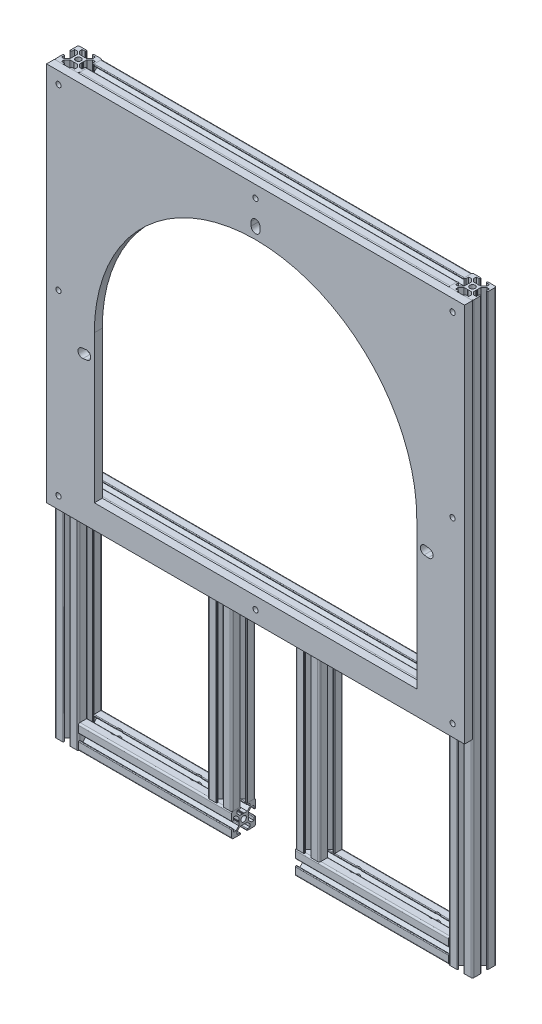
SolidWorks part; units mm, degrees
material "6061 合金"
ref_plane "前视基准面" through (0, 0, 0) normal (0, 0, 1) x (1, 0, 0)
ref_plane "上视基准面" through (0, 0, 0) normal (0, 1, 0) x (1, 0, 0)
ref_plane "右视基准面" through (0, 0, 0) normal (1, 0, 0) x (0, 0, -1)
sketch "草图2" plane through (0, 0, 0) normal (0, 0, 1) x (1, 0, 0)
  line L0 (0, 120) -> (0, 0) construction
  line L1 (262.5, 382.5) -> (-262.5, 382.5)
  line L2 (262.5, 382.5) -> (262.5, -600)
  line L3 (262.5, -600) -> (-262.5, -600)
  line L4 (-262.5, 382.5) -> (-262.5, -600)
  line L5 (0, 0) -> (-79.5734, 0) construction
  line L6 (-184, -30) -> (184, -30)
  line L7 (-184, -30) -> (-184, -525)
  line L8 (184, -30) -> (184, -525)
  circle A5 centre (0, 120) radius 242.5
  circle A6 centre (0, 120) radius 262.5
  point P7 (0, -600)
  dimension "D1" = 485
  dimension "D2" = 184
  dimension "D3" = 525
  dimension "D4" = 120
  dimension "D10" = 30
  dimension "D12" = 600
sketch "草图3" plane through (0, 0, 0) normal (0, 0, 1) x (1, 0, 0)
  line L0 (-247.5, -340) -> (-55, -340)
  line L1 (-247.5, 367.5) -> (247.5, 367.5)
  line L2 (-247.5, 367.5) -> (-247.5, -340)
  line L3 (-247.5, -80) -> (247.5, -80)
  line L4 (247.5, 367.5) -> (247.5, -340)
  line L5 (-55, -80) -> (-55, -340)
  line L6 (0, -22) -> (0, 22) construction
  line L7 (262.5, 382.5) -> (-262.5, 382.5) construction
  line L8 (262.5, 382.5) -> (262.5, -600) construction
  line L9 (-184, -30) -> (184, -30) construction
  line L10 (55, -80) -> (55, -340)
  line L11 (55, -340) -> (247.5, -340)
  point P8 (0, 367.5)
  dimension "D1" = 50
  dimension "D2" = 15
  dimension "D3" = 15
  dimension "D4" = 260
  dimension "D5" = 110
other "铝型材 30 X 30 X R2(1)"
ref_plane "基准面1" through (-247.5, 367.5, 0) normal (0, -1, 0) x (1, 0, 0)
sketch "草图1" plane through (-247.5, 367.5, 0) normal (0, -1, 0) x (1, 0, 0)
  line L0 (-15, -4.8) -> (-15, -13)
  line L1 (-13, -15) -> (-4.8, -15)
  line L2 (-4, -14.2) -> (-4, -13.8)
  line L3 (-4.8, -13) -> (-8.25, -13)
  line L4 (-8.25, -13) -> (-8.25, -9.6642)
  line L5 (-8.25, -9.6642) -> (-4.5858, -6)
  line L6 (-4.5858, -6) -> (-0.6536, -6)
  line L7 (-0.4036, -5.933) -> (0, -5.7)
  line L8 (0, -5.7) -> (0.4036, -5.933)
  line L9 (0.9036, -5.933) -> (1.2189, -5.751)
  line L10 (1.2189, -5.751) -> (2.5, -6)
  line L11 (2.5, -6) -> (4.5858, -6)
  line L12 (4.5858, -6) -> (8.25, -9.6642)
  line L13 (8.25, -9.6642) -> (8.25, -13)
  line L14 (8.25, -13) -> (4.8, -13)
  line L15 (4, -13.8) -> (4, -14.2)
  line L16 (4.8, -15) -> (13, -15)
  line L17 (15, -13) -> (15, -4.8)
  line L18 (14.2, -4) -> (13.8, -4)
  line L19 (13, -4.8) -> (13, -8.25)
  line L20 (13, -8.25) -> (9.6642, -8.25)
  line L21 (9.6642, -8.25) -> (6, -4.5858)
  line L22 (6, -4.5858) -> (6, -0.6536)
  line L23 (5.933, -0.4036) -> (5.7, 0)
  line L24 (5.7, 0) -> (5.933, 0.4036)
  line L25 (5.933, 0.9036) -> (5.751, 1.2189)
  line L26 (5.751, 1.2189) -> (6, 2.5)
  line L27 (6, 2.5) -> (6, 4.5858)
  line L28 (6, 4.5858) -> (9.6642, 8.25)
  line L29 (9.6642, 8.25) -> (13, 8.25)
  line L30 (13, 8.25) -> (13, 4.8)
  line L31 (13.8, 4) -> (14.2, 4)
  line L32 (15, 4.8) -> (15, 13)
  line L33 (13, 15) -> (4.8, 15)
  line L34 (4, 14.2) -> (4, 13.8)
  line L35 (4.8, 13) -> (8.25, 13)
  line L36 (8.25, 13) -> (8.25, 9.6642)
  line L37 (8.25, 9.6642) -> (4.5858, 6)
  line L38 (4.5858, 6) -> (0.6536, 6)
  line L39 (0.4036, 5.933) -> (0, 5.7)
  line L40 (0, 5.7) -> (-0.4036, 5.933)
  line L41 (-0.9036, 5.933) -> (-1.2189, 5.751)
  line L42 (-1.2189, 5.751) -> (-2.5, 6)
  line L43 (-2.5, 6) -> (-4.5858, 6)
  line L44 (-4.5858, 6) -> (-8.25, 9.6642)
  line L45 (-8.25, 9.6642) -> (-8.25, 13)
  line L46 (-8.25, 13) -> (-4.8, 13)
  line L47 (-4, 13.8) -> (-4, 14.2)
  line L48 (-4.8, 15) -> (-13, 15)
  line L49 (-15, 13) -> (-15, 4.8)
  line L50 (-14.2, 4) -> (-13.8, 4)
  line L51 (-13, 4.8) -> (-13, 8.25)
  line L52 (-13, 8.25) -> (-9.6642, 8.25)
  line L53 (-9.6642, 8.25) -> (-6, 4.5858)
  line L54 (-6, 4.5858) -> (-6, 0.6536)
  line L55 (-5.933, 0.4036) -> (-5.7, 0)
  line L56 (-5.7, 0) -> (-5.933, -0.4036)
  line L57 (-5.933, -0.9036) -> (-5.751, -1.2189)
  line L58 (-5.751, -1.2189) -> (-6, -2.5)
  line L59 (-6, -2.5) -> (-6, -4.5858)
  line L60 (-6, -4.5858) -> (-9.6642, -8.25)
  line L61 (-9.6642, -8.25) -> (-13, -8.25)
  line L62 (-13, -8.25) -> (-13, -4.8)
  line L63 (-13.8, -4) -> (-14.2, -4)
  arc A0 (-15, -13) -> (-13, -15) centre (-13, -13) ccw
  arc A1 (-4.8, -15) -> (-4, -14.2) centre (-4.8, -14.2) ccw
  arc A2 (-4, -13.8) -> (-4.8, -13) centre (-4.8, -13.8) ccw
  arc A3 (-0.6536, -6) -> (-0.4036, -5.933) centre (-0.6536, -5.5) ccw
  arc A4 (0.4036, -5.933) -> (0.9036, -5.933) centre (0.6536, -5.5) ccw
  arc A5 (4.8, -13) -> (4, -13.8) centre (4.8, -13.8) ccw
  arc A6 (4, -14.2) -> (4.8, -15) centre (4.8, -14.2) ccw
  arc A7 (13, -15) -> (15, -13) centre (13, -13) ccw
  arc A8 (15, -4.8) -> (14.2, -4) centre (14.2, -4.8) ccw
  arc A9 (13.8, -4) -> (13, -4.8) centre (13.8, -4.8) ccw
  arc A10 (6, -0.6536) -> (5.933, -0.4036) centre (5.5, -0.6536) ccw
  arc A11 (5.933, 0.4036) -> (5.933, 0.9036) centre (5.5, 0.6536) ccw
  arc A12 (13, 4.8) -> (13.8, 4) centre (13.8, 4.8) ccw
  arc A13 (14.2, 4) -> (15, 4.8) centre (14.2, 4.8) ccw
  arc A14 (15, 13) -> (13, 15) centre (13, 13) ccw
  arc A15 (4.8, 15) -> (4, 14.2) centre (4.8, 14.2) ccw
  arc A16 (4, 13.8) -> (4.8, 13) centre (4.8, 13.8) ccw
  arc A17 (0.6536, 6) -> (0.4036, 5.933) centre (0.6536, 5.5) ccw
  arc A18 (-0.4036, 5.933) -> (-0.9036, 5.933) centre (-0.6536, 5.5) ccw
  arc A19 (-4.8, 13) -> (-4, 13.8) centre (-4.8, 13.8) ccw
  arc A20 (-4, 14.2) -> (-4.8, 15) centre (-4.8, 14.2) ccw
  arc A21 (-13, 15) -> (-15, 13) centre (-13, 13) ccw
  arc A22 (-15, 4.8) -> (-14.2, 4) centre (-14.2, 4.8) ccw
  arc A23 (-13.8, 4) -> (-13, 4.8) centre (-13.8, 4.8) ccw
  arc A24 (-6, 0.6536) -> (-5.933, 0.4036) centre (-5.5, 0.6536) ccw
  arc A25 (-5.933, -0.4036) -> (-5.933, -0.9036) centre (-5.5, -0.6536) ccw
  arc A26 (-13, -4.8) -> (-13.8, -4) centre (-13.8, -4.8) ccw
  arc A27 (-14.2, -4) -> (-15, -4.8) centre (-14.2, -4.8) ccw
  circle A28 centre (0, 0) radius 3.4
  point P123 (0, 0)
  dimension "D3" = 6.8
  dimension "D1" = 30
  dimension "D2" = 30
sketch "草图5" plane through (0, 189.5603, 15) normal (0, 0, -1) x (-1, 0, 0)
  line L1 (262.5, 192.9397) -> (-262.5, 192.9397)
  line L2 (262.5, 192.9397) -> (262.5, -284.5603)
  line L3 (262.5, -284.5603) -> (-262.5, -284.5603)
  line L4 (-262.5, 192.9397) -> (-262.5, -284.5603)
  line L6 (-202.5, -254.5603) -> (202.5, -254.5603)
  line L7 (-262.5, 192.9397) -> (-262.5, -789.5603) construction
  line L8 (-202.5, -69.5603) -> (-202.5, -254.5603)
  line L9 (202.5, -69.5603) -> (202.5, -254.5603)
  line L10 (262.5, 192.9397) -> (262.5, -789.5603) construction
  line L13 (-232.5, -254.5603) -> (232.5, -254.5603) construction
  arc A0 (202.5, -69.5603) -> (-202.5, -69.5603) centre (0, -69.5603) ccw
  circle A1 centre (0, -69.5603) radius 242.5 construction
  dimension "D1" = 40
extrude "凸台-拉伸1" add sketch "草图5" against normal blind 10 separate body
sketch "草图6" plane through (0, 0, 25) normal (0, 0, 1) x (1, 0, 0)
  line L0 (0, 339.5) -> (0, 334.5) construction
  line L1 (5.5, 339.5) -> (5.5, 334.5)
  line L2 (-5.5, 339.5) -> (-5.5, 334.5)
  line L3 (-217.477, 90.2675) -> (-212.523, 90.9448) construction
  line L5 (-218.222, 95.7168) -> (-213.268, 96.3941)
  line L6 (-216.732, 84.8182) -> (-211.778, 85.4955)
  line L7 (-215, 90.6061) -> (0, 120) construction
  line L8 (0, -22) -> (0, 22) construction
  line L9 (217.477, 90.2675) -> (212.523, 90.9448) construction
  line L10 (218.222, 95.7168) -> (213.268, 96.3941)
  line L11 (216.732, 84.8182) -> (211.778, 85.4955)
  circle A0 centre (0, 120) radius 217 construction
  arc A1 (5.5, 339.5) -> (-5.5, 339.5) centre (0, 339.5) ccw
  arc A2 (-5.5, 334.5) -> (5.5, 334.5) centre (0, 334.5) ccw
  arc A3 (-218.222, 95.7168) -> (-216.732, 84.8182) centre (-217.477, 90.2675) ccw
  arc A4 (-211.778, 85.4955) -> (-213.268, 96.3941) centre (-212.523, 90.9448) ccw
  arc A5 (218.222, 95.7168) -> (216.732, 84.8182) centre (217.477, 90.2675) cw
  arc A6 (211.778, 85.4955) -> (213.268, 96.3941) centre (212.523, 90.9448) cw
  point P5 (0, 337)
  point P15 (-215, 90.6061)
  point P24 (215, 90.6061)
  dimension "D1" = 434
  dimension "D2" = 11
  dimension "D3" = 5
  dimension "D4" = 11
  dimension "D5" = 5
  dimension "D6" = 430
extrude "切除-拉伸1" cut sketch "草图6" against normal up to next (10 mm away)
sketch "草图7" plane through (0, 0, 25) normal (0, 0, 1) x (1, 0, 0)
  line L0 (-262.5, 143.75) -> (262.5, 143.75) construction
  line L1 (-262.5, -95) -> (-262.5, 382.5) construction
  line L2 (262.5, 382.5) -> (262.5, -95) construction
  line L3 (0, -95) -> (0, 143.75) construction
  line L4 (262.5, -95) -> (-262.5, -95) construction
  line L5 (-262.5, 382.5) -> (262.5, 382.5) construction
  circle A0 centre (-247.5, 367.5) radius 3.25
  circle A1 centre (0, 367.5) radius 3.25
  circle A2 centre (-247.5, 143.75) radius 3.25
  circle A3 centre (0, -80) radius 3.25
  circle A4 centre (-247.5, -80) radius 3.25
  circle A5 centre (247.5, 143.75) radius 3.25
  circle A6 centre (247.5, 367.5) radius 3.25
  circle A7 centre (247.5, -80) radius 3.25
  dimension "D1" = 6.5
  dimension "D2" = 15
  dimension "D3" = 15
extrude "切除-拉伸2" cut sketch "草图7" against normal up to next (10 mm away)
other "剪裁/延伸1" [suppressed]
other "剪裁/延伸2" [suppressed]
ref_plane "基准面2" through (0, -80, 0) normal (0, 1, 0) x (1, 0, 0)
sketch "草图8" plane through (0, -325, 0) normal (0, 1, 0) x (1, 0, 0)
  line L0 (0, -22) -> (0, 22) construction
  line L1 (55, 0) -> (247.5, 0) construction
  circle A1 centre (100, 0) radius 5.5
  circle A2 centre (200, 0) radius 5.5
  circle A3 centre (-200, 0) radius 5.5
  circle A4 centre (-100, 0) radius 5.5
  dimension "D1" = 11
  dimension "D3" = 400
  dimension "D4" = 100
  dimension "D2" = 2
extrude "切除-拉伸3" cut sketch "草图8" against normal through all
